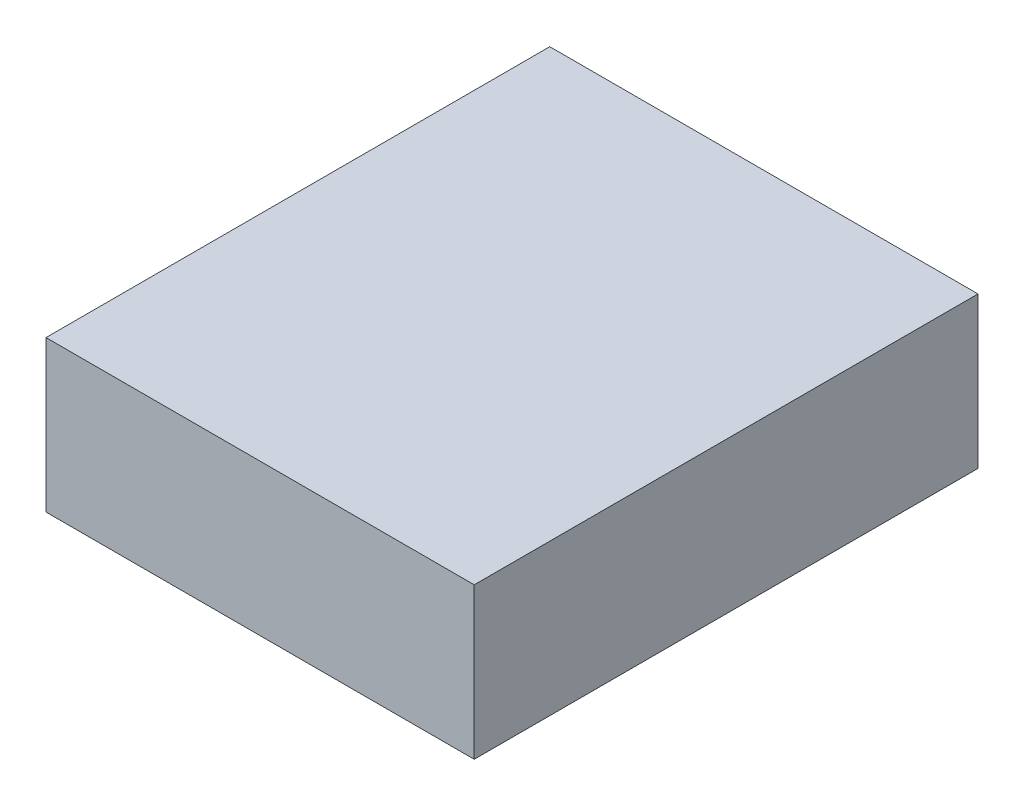
SolidWorks part; units mm, degrees
material "AISI 1015 钢，冷拔 (SS)"
ref_plane "Front Plane" through (0, 0, 0) normal (0, 0, 1) x (1, 0, 0)
ref_plane "Top Plane" through (0, 0, 0) normal (0, 1, 0) x (1, 0, 0)
ref_plane "Right Plane" through (0, 0, 0) normal (1, 0, 0) x (0, 0, -1)
other "Configuration Table"
sketch "Sketch1" plane through (0, 0, 0) normal (1, 0, 0) x (0, 0, -1)
  line L1 (0, 0) -> (100, 0)
  line L2 (0, 0) -> (0, 30)
  line L3 (0, 30) -> (100, 30)
  line L4 (100, 0) -> (100, 30)
  dimension "D1" = 100
  dimension "D2" = 30
extrude "Boss-Extrude1" add sketch "Sketch1" along normal blind 85
